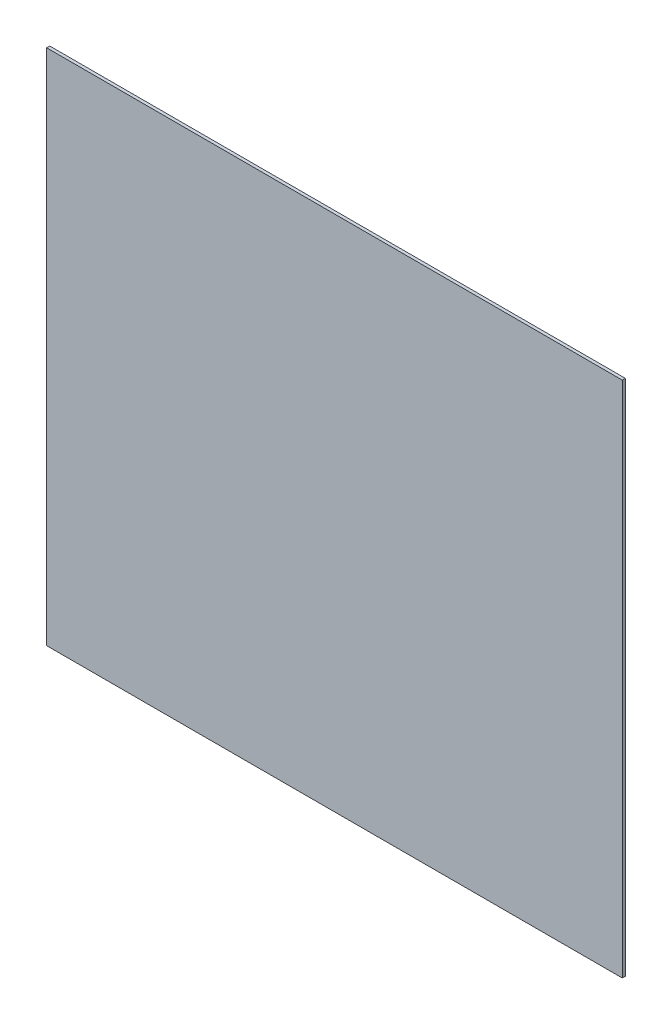
SolidWorks part; units mm, degrees
material "PMMA(有机玻璃)"
ref_plane "前视" through (0, 0, 0) normal (0, 0, 1) x (1, 0, 0)
ref_plane "上视" through (0, 0, 0) normal (0, 1, 0) x (1, 0, 0)
ref_plane "右视" through (0, 0, 0) normal (1, 0, 0) x (0, 0, -1)
sketch "草图1" plane through (0, 0, 0) normal (0, 0, 1) x (1, 0, 0)
  line L1 (-468, 421) -> (468, 421)
  line L2 (-468, 421) -> (-468, -421)
  line L3 (-468, -421) -> (468, -421)
  line L4 (468, 421) -> (468, -421)
  line L5 (-468, 421) -> (468, -421) construction
  line L6 (-468, -421) -> (468, 421) construction
  point P0 (0, 0)
  dimension "D1" = 842
  dimension "D2" = 936
extrude "凸台-拉伸1" add sketch "草图1" along normal blind 5
hole_wizard "M5 间隙孔1" positions "草图3" profile "草图2" hole size "M5" standard "GB"
sketch "草图3" plane through (0, 0, 5) normal (0, 0, 1) x (1, 0, 0)
  line L0 (-427.5, 273) -> (-427.5, -273) construction
  line L1 (-427.5, -273) -> (427.5, -273) construction
  line L2 (0, 273) -> (0, -273) construction
  line L3 (427.5, 273) -> (-427.5, 273) construction
  line L5 (-427.5, 0) -> (427.5, 0) construction
  line L6 (427.5, -273) -> (427.5, 273) construction
  point P0 (-375, -261)
  point P46 (415.5, 250)
  point P48 (-415.5, 250)
  point P58 (-125, -261)
  point P59 (125, -261)
  point P61 (-125, 261)
  point P62 (125, 261)
  point P64 (-375, 261)
  point P88 (375, -261)
  point P89 (375, 261)
  point P108 (415.5, 0)
  point P109 (-415.5, 0)
  point P110 (415.5, -250)
  point P111 (-415.5, -250)
  dimension "D1" = 12
  dimension "D2" = 12
  dimension "D5" = 3
  dimension "D3" = 12
  dimension "D6" = 4
  dimension "D4" = 2
sketch "草图2" plane through (-375, -261, 5) normal (1, 0, 0) x (0, -1, 0)
  line L0 (0, 0) -> (0, 5)
  line L1 (0, 5) -> (2.75, 5)
  line L2 (2.75, 5) -> (2.75, 0)
  line L5 (2.75, 0) -> (0, 0)
  line L11 (0, -6.35) -> (0, 107.95) construction
  dimension "通孔孔直径" = 5.5
  dimension "通孔孔深度" = 5
